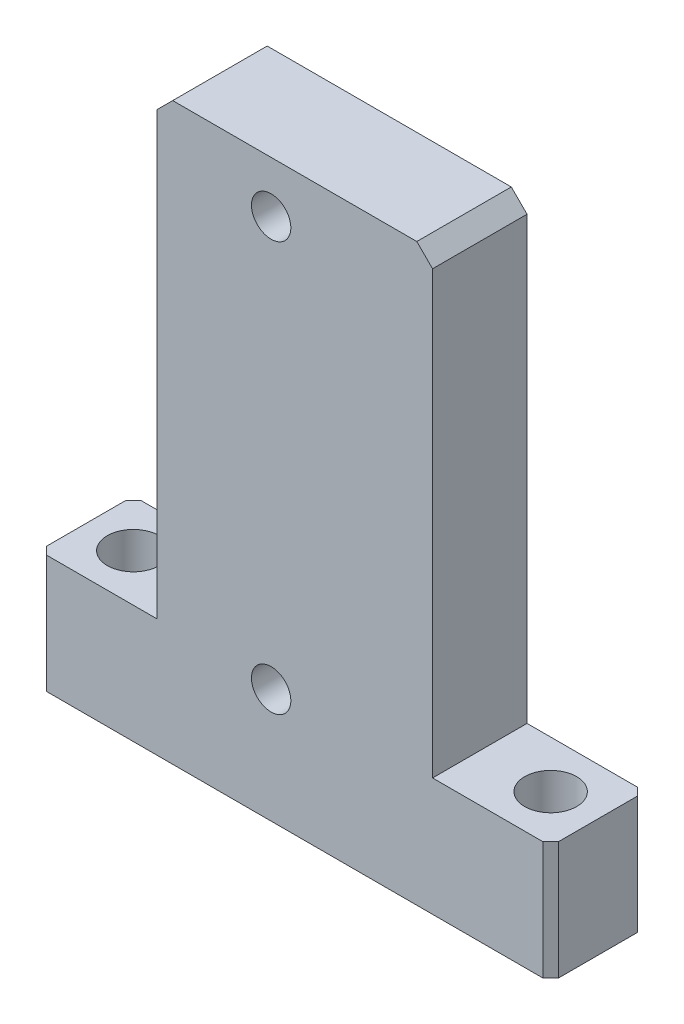
from build123d import *

# Parameters (mm, degrees)
SKETCH_1_W           = 35
SKETCH_1_H           = 73
EXTRUDE_1_DEPTH      = 6
SKETCH_2_W           = 65
SKETCH_2_H           = 12
EXTRUDE_2_DEPTH      = 15
HOLE_WIZARD_M6_1_D   = 6.6
F_6_0MM_1_D          = 6
F_6_0MM_1_DEPTH      = 15
F_6_0MM_1_TIP        = 1.802581857
HOLE_WIZARD_M6_1_2_D = 5
CHAMFER_1_SIZE       = 1
CHAMFER_2_SIZE       = 2


with BuildPart() as part:
    # 草图1 → 凸台-拉伸1 (new, symmetric)
    with BuildSketch(Plane.XY):
        Rectangle(SKETCH_1_W, SKETCH_1_H)
    extrude(amount=EXTRUDE_1_DEPTH, both=True)

    # 草图2 → 凸台-拉伸2 (add)
    with BuildSketch(Plane.XZ.offset(36.5)):
        Rectangle(SKETCH_2_W, SKETCH_2_H)
    extrude(amount=-EXTRUDE_2_DEPTH)

    # Hole Wizard M6 _1 (through all)
    with Locations(Plane(origin=(0, -21.5, 0), x_dir=(1, 0, 0), z_dir=(0, 1, 0))):
        with Locations((-26.5, 0), (26.5, 0)):
            Hole(HOLE_WIZARD_M6_1_D / 2)

    # Ø6.0mm 暗销孔1
    with Locations(Plane(origin=(0, -36.5, 0), x_dir=(-1, 0, 0), z_dir=(0, -1, 0))):
        with Locations((10, 0), (-10, 0)):
            Hole(F_6_0MM_1_D / 2, depth=F_6_0MM_1_DEPTH)
            with Locations((0, 0, -(F_6_0MM_1_DEPTH + F_6_0MM_1_TIP / 2))):  # 118° drill point
                Cone(0, F_6_0MM_1_D / 2, F_6_0MM_1_TIP, mode=Mode.SUBTRACT)

    # Hole Wizard M6 _1 2 (through all)
    with Locations(Plane(origin=(0, 0, -6), x_dir=(-1, 0, 0), z_dir=(0, 0, -1))):
        with Locations((3, -22), (3, 30)):
            Hole(HOLE_WIZARD_M6_1_2_D / 2)

    # 倒角1
    chamfer_1_edges = [part.edges().sort_by_distance(p)[0] for p in [
        (-32.5, -29, 6),
        (32.5, -29, -6),
        (-32.5, -29, -6),
        (32.5, -29, 6),
    ]]
    chamfer(chamfer_1_edges, length=CHAMFER_1_SIZE)

    # 倒角2
    chamfer_2_edges = [part.edges().sort_by_distance(p)[0] for p in [
        (-17.5, 36.5, 0),
        (17.5, 36.5, 0),
    ]]
    chamfer(chamfer_2_edges, length=CHAMFER_2_SIZE)


solid = part.part
